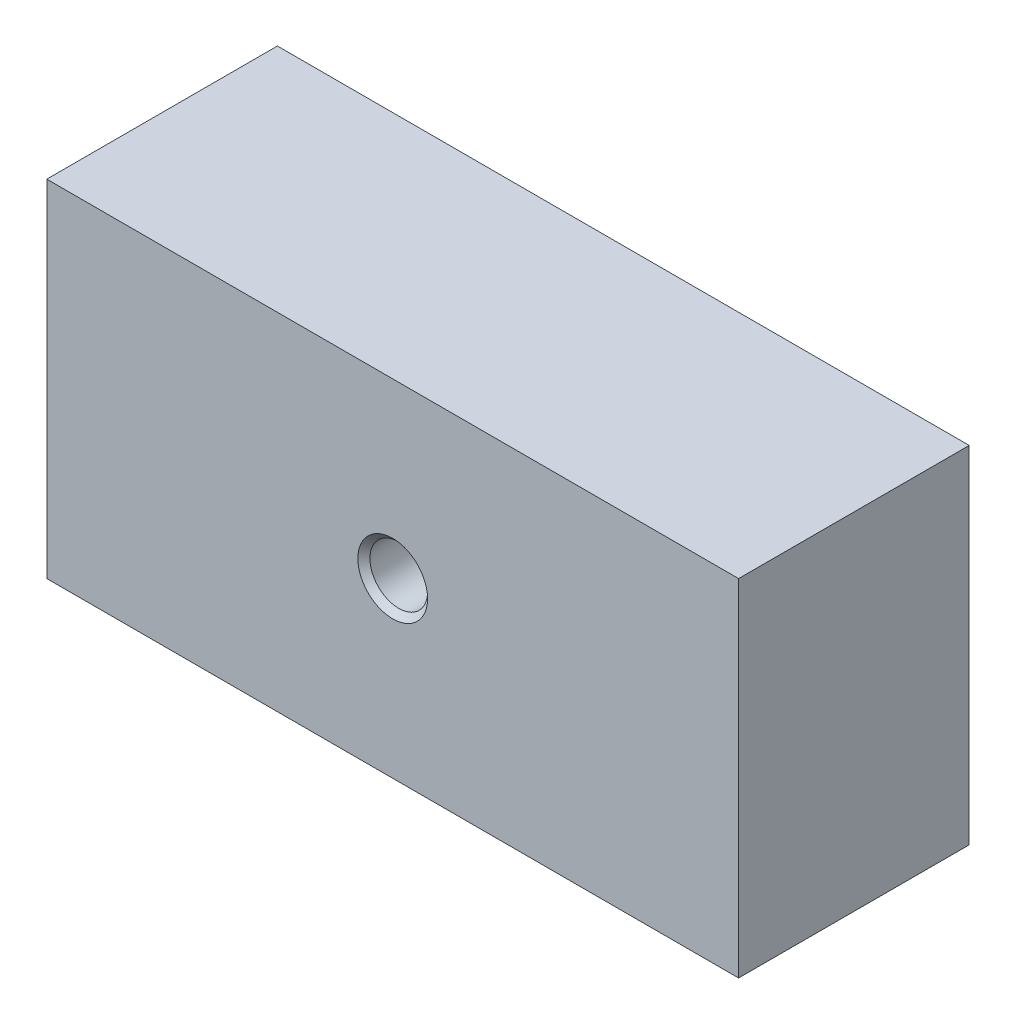
from build123d import *

# Parameters (mm, degrees)
SKETCH1_W                   = 60
SKETCH1_H                   = 30
BOSS_EXTRUDE1_DEPTH         = 20
M6_TAPPED_HOLE1_D           = 5
M6_TAPPED_HOLE1_DEPTH       = 15
M6_TAPPED_HOLE1_CSINK_D     = 6.05
M6_TAPPED_HOLE1_CSINK_ANGLE = 90
M6_TAPPED_HOLE1_TIP         = 1.502151548


with BuildPart() as part:
    # Sketch1 → Boss-Extrude1 (new body)
    with BuildSketch(Plane.XY):
        with Locations((720, 45)):
            Rectangle(SKETCH1_W, SKETCH1_H)
    extrude(amount=BOSS_EXTRUDE1_DEPTH)

    # M6 Tapped Hole1
    with Locations(Plane.XY.offset(20)):
        with Locations((720, 45)):
            CounterSinkHole(M6_TAPPED_HOLE1_D / 2, M6_TAPPED_HOLE1_CSINK_D / 2, depth=M6_TAPPED_HOLE1_DEPTH, counter_sink_angle=M6_TAPPED_HOLE1_CSINK_ANGLE)
            with Locations((0, 0, -(M6_TAPPED_HOLE1_DEPTH + M6_TAPPED_HOLE1_TIP / 2))):  # 118° drill point
                Cone(0, M6_TAPPED_HOLE1_D / 2, M6_TAPPED_HOLE1_TIP, mode=Mode.SUBTRACT)


solid = part.part
